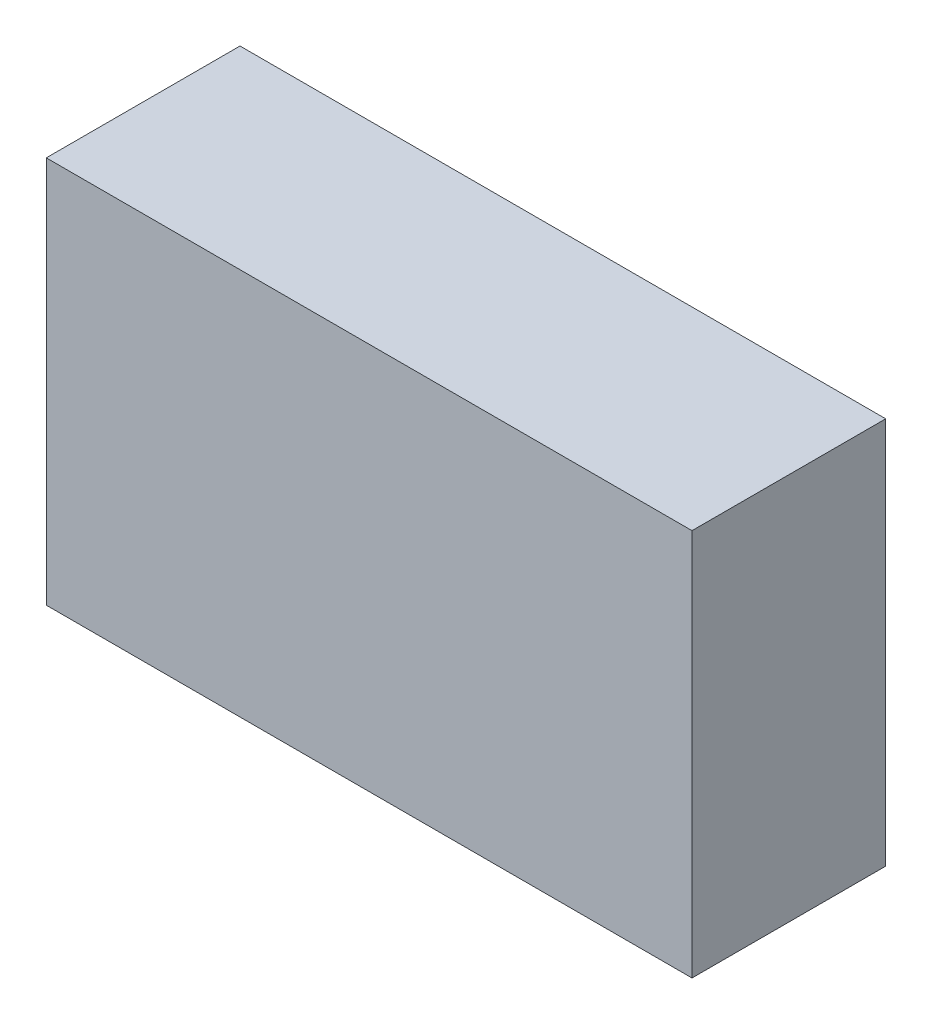
from build123d import *

# Parameters (mm, degrees)
SKETCH1_W           = 100
SKETCH1_H           = 60
BOSS_EXTRUDE1_DEPTH = 30


with BuildPart() as part:
    # Sketch1 → Boss-Extrude1 (new body)
    with BuildSketch(Plane.XY):
        Rectangle(SKETCH1_W, SKETCH1_H)
    extrude(amount=BOSS_EXTRUDE1_DEPTH)


solid = part.part
